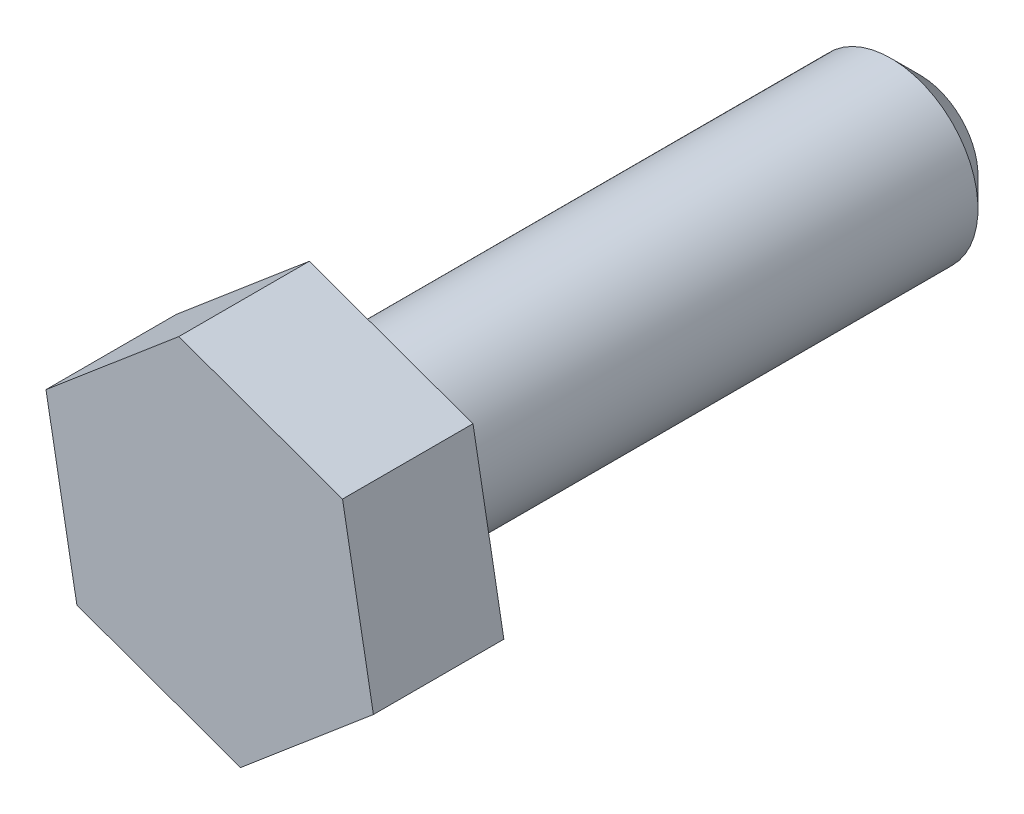
SolidWorks part; units mm, degrees
ref_plane "Front Plane" through (0, 0, 0) normal (0, 0, 1) x (1, 0, 0)
ref_plane "Top Plane" through (0, 0, 0) normal (0, 1, 0) x (1, 0, 0)
ref_plane "Right Plane" through (0, 0, 0) normal (1, 0, 0) x (0, 0, -1)
sketch "Sketch1" plane through (0, 0, 0) normal (0, 0, 1) x (1, 0, 0)
  circle A0 centre (0, 0) radius 6
  dimension "D1" = 12
extrude "Boss-Extrude1" add sketch "Sketch1" along normal blind 4.5
sketch "Sketch2" plane through (0, 0, 0) normal (0, 0, -1) x (-1, 0, 0)
  line L1 (4.5811, -3.8747) -> (5.6461, 2.03)
  line L2 (5.6461, 2.03) -> (1.065, 5.9047)
  line L3 (1.065, 5.9047) -> (-4.5811, 3.8747)
  line L4 (-4.5811, 3.8747) -> (-5.6461, -2.03)
  line L5 (-5.6461, -2.03) -> (-1.065, -5.9047)
  line L6 (-1.065, -5.9047) -> (4.5811, -3.8747)
  circle A0 centre (0, 0) radius 5.1962 construction
extrude "Cut-Extrude1" cut sketch "Sketch2" against normal blind 4.5 flip side to cut
sketch "Sketch3" plane through (0, 0, 0) normal (0, 0, -1) x (-1, 0, 0)
  circle A0 centre (0, 0) radius 3
  dimension "D1" = 6
extrude "Boss-Extrude2" add sketch "Sketch3" along normal blind 20
cosmetic thread "Cosmetic Thread1" parameters "D2"=5
chamfer "Chamfer2" distance 1 angle 45 1 edges at (-3, 0, -20)
